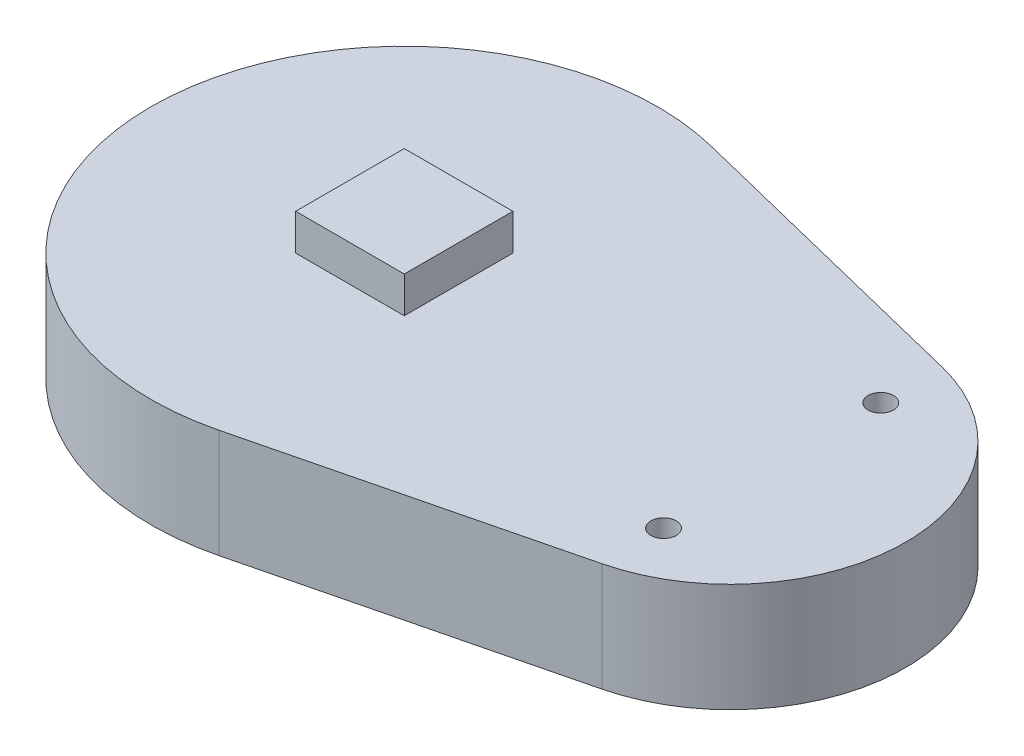
SolidWorks part; units mm, degrees
ref_plane "Front Plane" through (0, 0, 0) normal (0, 0, 1) x (1, 0, 0)
ref_plane "Top Plane" through (0, 0, 0) normal (0, 1, 0) x (1, 0, 0)
ref_plane "Right Plane" through (0, 0, 0) normal (1, 0, 0) x (0, 0, -1)
sketch "Sketch1" plane through (0, 0, 0) normal (0, 1, 0) x (1, 0, 0)
  line L0 (0, 0) -> (0, 109) construction
  line L1 (0, 109) -> (-90, 109) construction
  line L2 (11.61, 0) -> (11.61, 62) construction
  line L3 (-73.2099, 176.9565) -> (11.6122, 155.9995)
  line L4 (-73.2099, 41.0435) -> (11.6122, 62.0005)
  circle A0 centre (-90, 109) radius 70 construction
  circle A1 centre (0, 109) radius 48.4127 construction
  arc A2 (-73.2099, 176.9565) -> (-73.2099, 41.0435) centre (-90, 109) ccw
  arc A3 (11.61, 62) -> (11.6122, 155.9995) centre (0, 109) ccw
  dimension "D3" = 140
  dimension "D1" = 109
  dimension "D2" = 90
  dimension "D4" = 62
  dimension "D5" = 11.61
extrude "Boss-Extrude1" add sketch "Sketch1" along normal blind 30 contours L4 A3 L3 A2
sketch "Sketch2" plane through (0, 30, 0) normal (0, 1, 0) x (1, 0, 0)
  line L1 (-105, 124) -> (-75, 124)
  line L2 (-105, 124) -> (-105, 94)
  line L3 (-105, 94) -> (-75, 94)
  line L4 (-75, 124) -> (-75, 94)
  line L5 (-105, 124) -> (-75, 94) construction
  line L6 (-105, 94) -> (-75, 124) construction
  arc A0 (-73.2099, 176.9565) -> (-73.2099, 41.0435) centre (-90, 109) ccw construction
  arc A1 (-73.2099, 176.9565) -> (-73.2099, 41.0435) centre (-90, 109) ccw construction
  dimension "D1" = 30
  dimension "D2" = 30
extrude "Boss-Extrude2" add sketch "Sketch2" along normal blind 10
sketch "Sketch3" plane through (0, 0, 0) normal (0, -1, 0) x (1, 0, 0)
  circle A0 centre (-90, -109) radius 65
  dimension "D1" = 130
extrude "Boss-Extrude3" add sketch "Sketch3" along normal blind 3.01
sketch "Sketch4" plane through (0, -3.01, 0) normal (0, -1, 0) x (1, 0, 0)
  circle A0 centre (-90, -109) radius 30
  dimension "D1" = 60
extrude "Boss-Extrude4" add sketch "Sketch4" along normal blind 8 contours A0
sketch "Sketch5" plane through (0, 0, 0) normal (0, -1, 0) x (1, 0, 0)
  line L0 (-160, -109) -> (48.4127, -109) construction
  arc A0 (-73.2099, -41.0435) -> (-73.2099, -176.9565) centre (-90, -109) ccw construction
  arc A1 (11.6122, -155.9995) -> (11.6122, -62.0005) centre (0, -109) ccw construction
  point P0 (11.6122, -79)
  point P1 (11.6122, -139)
  dimension "D1" = 60
hole_wizard "CBORE for M6 Pan Head Screw1" positions "3DSketch1" profile "Sketch6" counterbore size "M6" standard "ISO"
sketch3d "3DSketch1"
  point P0 (11.6122, 0, -79)
  point P3 (11.6122, 0, -139)
sketch "Sketch6" plane through (11.6122, 0, -79) normal (1, 0, 0) x (0, 0, -1)
  line L0 (0, 0) -> (0, 52.603)
  line L1 (0, 52.603) -> (3.5, 50.5)
  line L2 (3.5, 50.5) -> (3.5, 4.6)
  line L3 (3.5, 4.6) -> (6.5, 4.6)
  line L4 (6.5, 4.6) -> (6.5, 0)
  line L5 (6.5, 0) -> (0, 0)
  line L10 (0, 52.603) -> (-3.5, 50.5) construction
  line L11 (0, -6.35) -> (0, 107.95) construction
  dimension "Hole Dia." = 7
  dimension "Hole Depth" = 50.5
  dimension "C'Bore Dia." = 13
  dimension "C'Bore Depth" = 4.6
  dimension "Drill Angle" = 118
sketch "Sketch7" plane through (0, 30, 0) normal (0, 1, 0) x (1, 0, 0)
  line L2 (-73.2099, 41.0435) -> (11.6122, 62.0005)
  line L3 (11.6122, 155.9995) -> (-73.2099, 176.9565)
  line L4 (-73.2099, 41.0435) -> (11.6122, 62.0005)
  line L5 (11.6122, 155.9995) -> (-73.2099, 176.9565)
  arc A2 (11.6122, 62.0005) -> (11.6122, 155.9995) centre (0, 109) ccw
  arc A3 (-73.2099, 176.9565) -> (-73.2099, 41.0435) centre (-90, 109) ccw
  arc A4 (11.6122, 62.0005) -> (11.6122, 155.9995) centre (0, 109) ccw
  arc A5 (-73.2099, 176.9565) -> (-73.2099, 41.0435) centre (-90, 109) ccw
  dimension "D1" = 0
